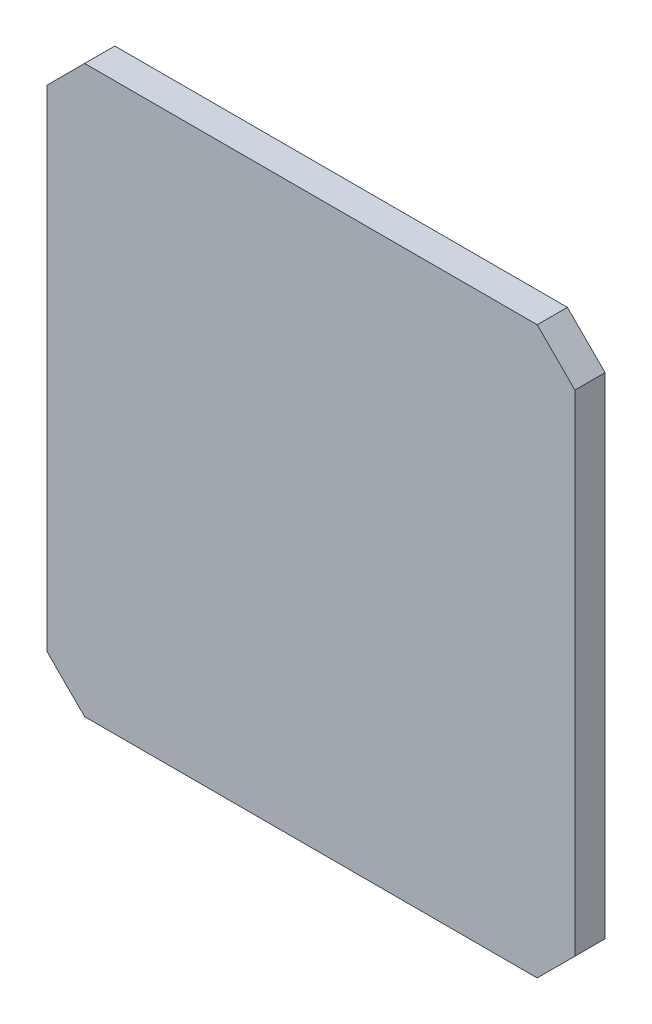
from build123d import *

# Parameters (mm, degrees)
EXTRUDE_1_DEPTH = 40


with BuildPart() as part:
    # 草图2 → 凸台-拉伸1 (new body)
    with BuildSketch(Plane.XY):
        Polygon((0, 700), (50, 750), (650, 750), (700, 700), (700, 50), (650, 0), (50, 0), (0, 50), align=None)
    extrude(amount=EXTRUDE_1_DEPTH)


solid = part.part
